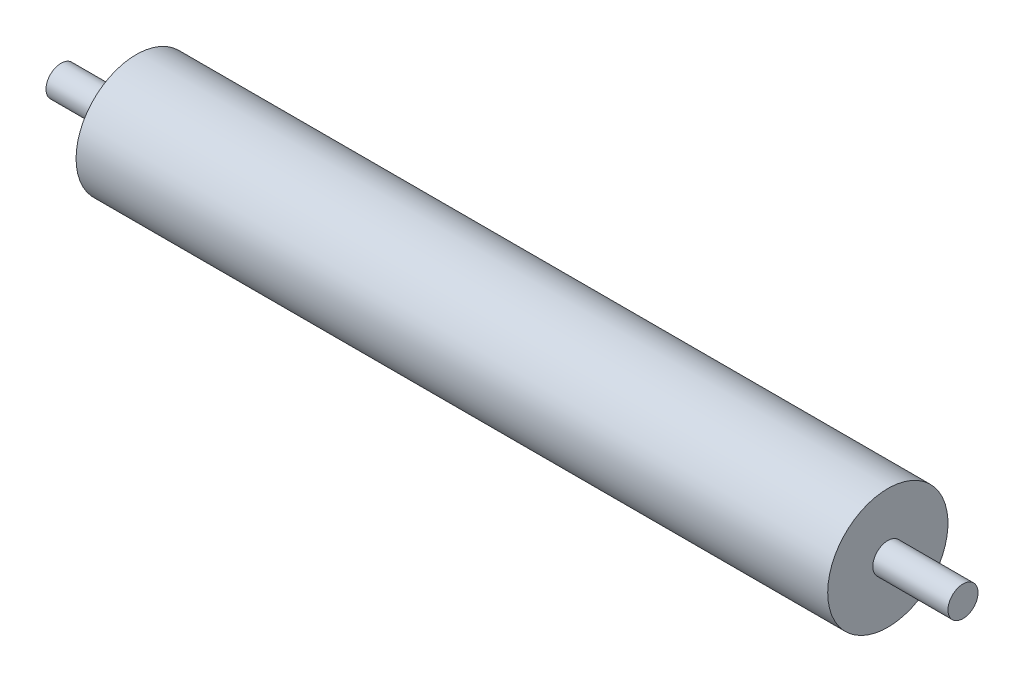
SolidWorks part; units mm, degrees
material "普通碳钢"
ref_plane "Front Plane" through (0, 0, 0) normal (0, 0, 1) x (1, 0, 0)
ref_plane "Top Plane" through (0, 0, 0) normal (0, 1, 0) x (1, 0, 0)
ref_plane "Right Plane" through (0, 0, 0) normal (1, 0, 0) x (0, 0, -1)
sketch "Sketch1" plane through (0, 0, 0) normal (0, 0, 1) x (1, 0, 0)
  line L0 (-223.0246, 190.4137) -> (376.9754, 190.4137)
  line L1 (376.9754, 190.4137) -> (376.9754, 200.4137)
  line L2 (376.9754, 200.4137) -> (326.9754, 200.4137)
  line L3 (326.9754, 200.4137) -> (326.9754, 230.4137)
  line L4 (326.9754, 230.4137) -> (-173.0246, 230.4137)
  line L5 (-173.0246, 230.4137) -> (-173.0246, 200.4137)
  line L6 (-173.0246, 200.4137) -> (-223.0246, 200.4137)
  line L7 (-223.0246, 200.4137) -> (-223.0246, 190.4137)
  dimension "D1" = 10
  dimension "D2" = 10
  dimension "D3" = 50
  dimension "D4" = 50
  dimension "D5" = 40
  dimension "D6" = 500
revolve "Revolve1" add sketch "Sketch1" angle 360 about L0
